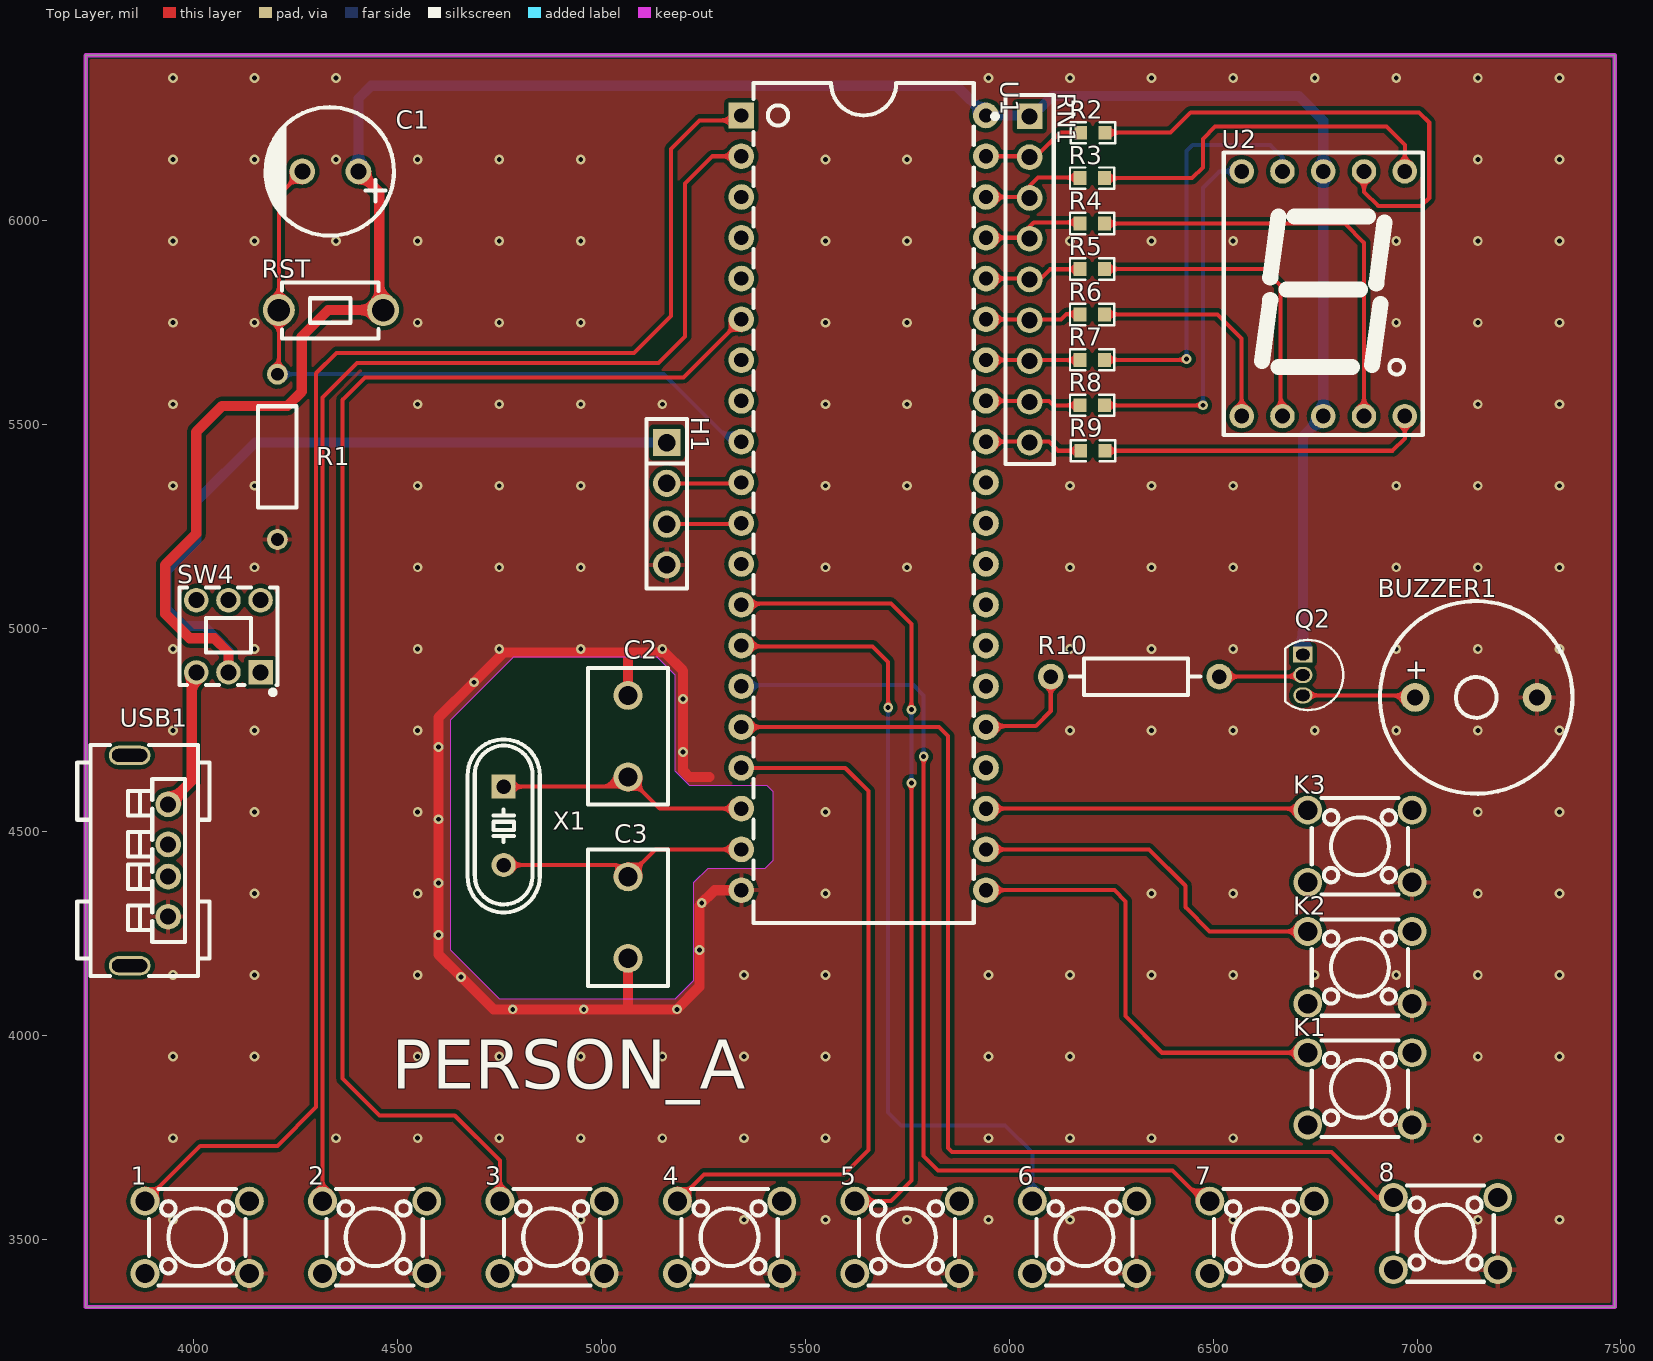
[diagram p0: Top Layer view]
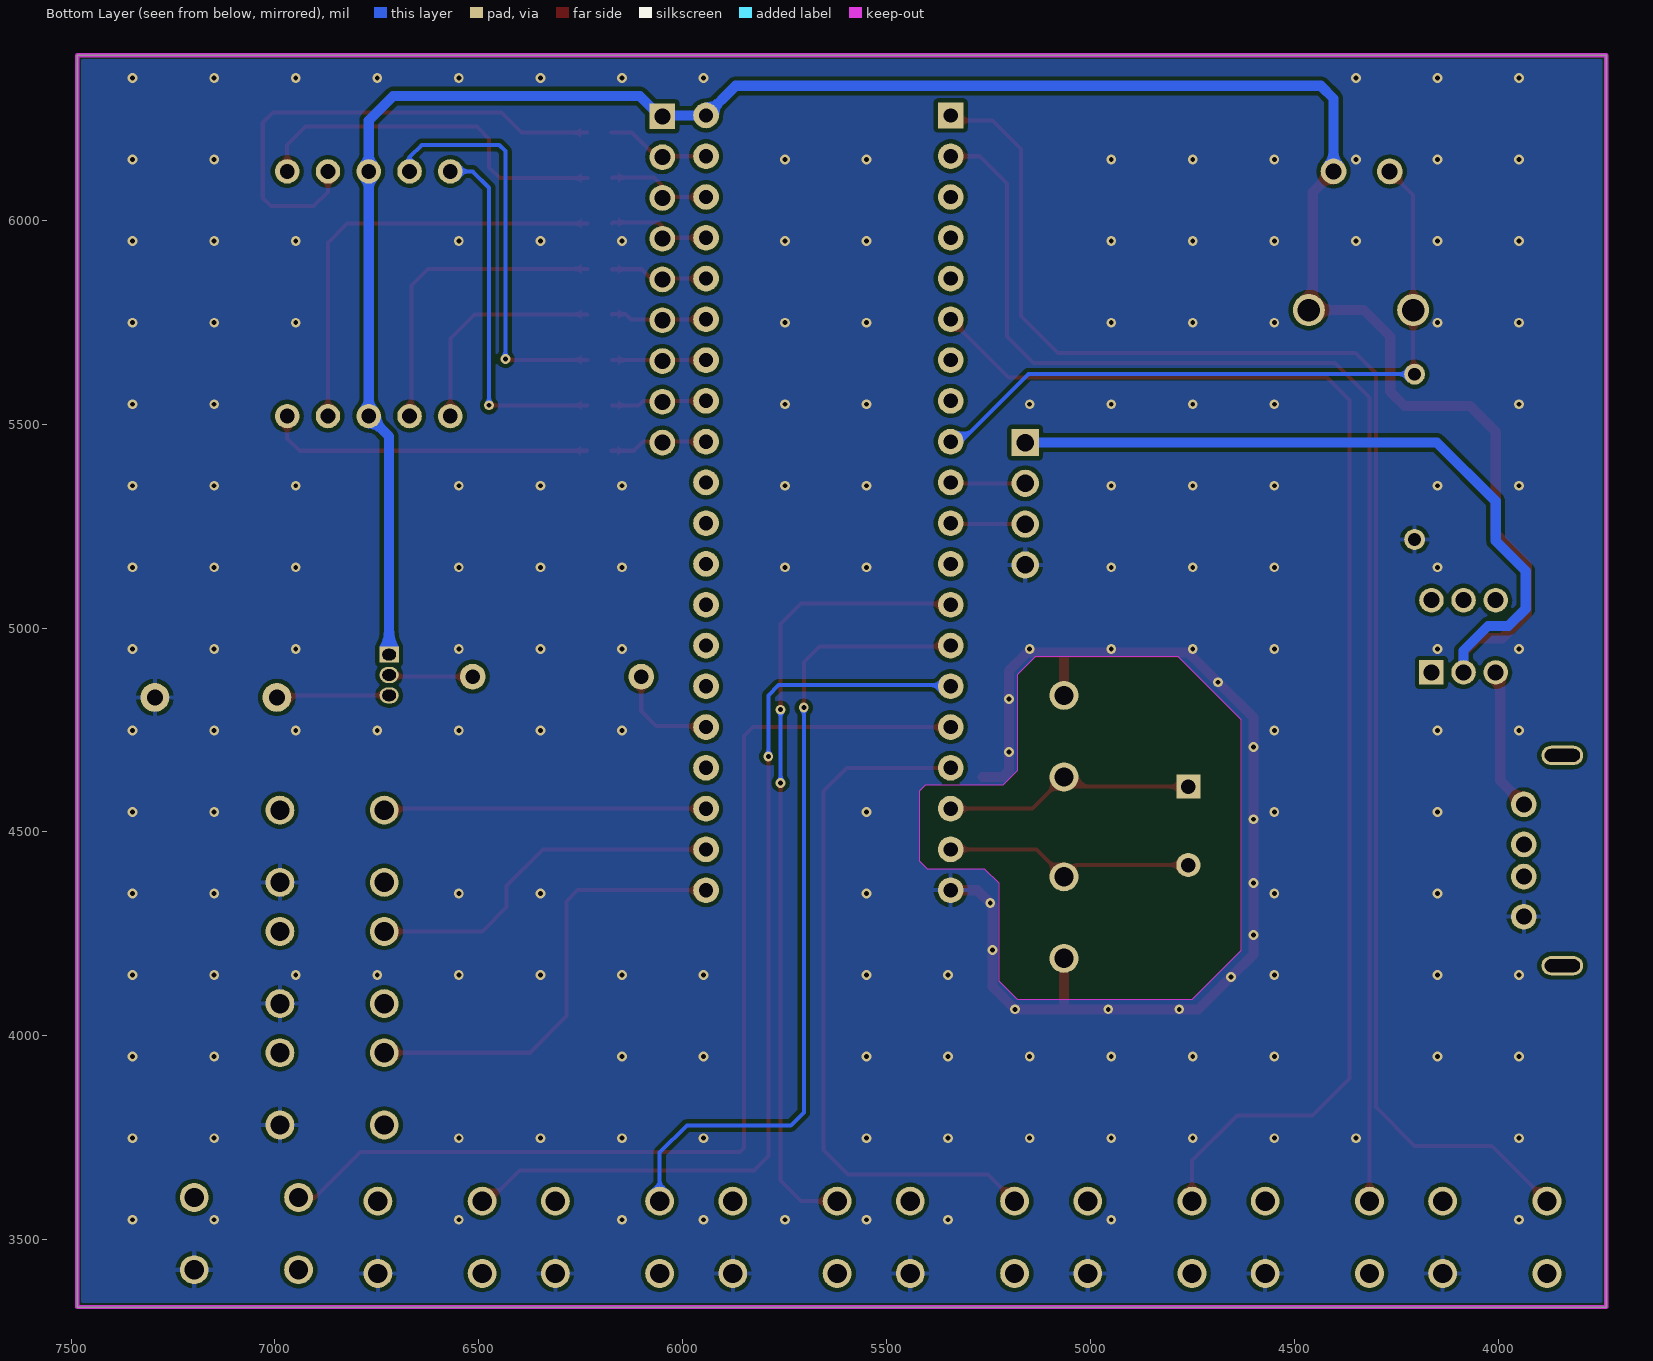
[diagram p1: Bottom Layer view, seen from below]
# Altium PCB MISC49928.pcbdoc
Units mil, origin at the board's own origin, x right, y up, seen from the top; angles counter-clockwise.
Board outline 3750 x 3070 mil, 2 copper layers (Top Layer, Bottom Layer), stack 62.206 mil thick; 34 components, 38 nets, 154 pads, 181 vias.

## Layer stack, top to bottom
Top Solder Mask Layer: solder mask 0.394, Dk 3.3
Top Layer: signal copper 1.379
Dielectric1: surface 59.449, FR4, Dk 4.5
Bottom Layer: signal copper 1.378
Bottom Solder Mask Layer: solder mask 0.394, Dk 3.3

## Board outline
3735,6405 3735,3335 7485,3335 7485,6405

## Design rules (kind name [scope] priority, off if disabled: settings)
BoardOutlineClearance copperThickness2oz_1 [All] p2 off: genericclearance=7.99 ignorepadtopadclearanceinfootprint=FALSE except(0: Arc-SplitContinuation Track-SplitContinuation SMDPad-SplitContinuation THPad-SplitContinuation Via-SplitContinuation Fill-SplitContinuation Region-SplitContinuation Poly-SplitContinuation Text-SplitContinuation Hole-SplitContinuation; 5.98: Arc-CutoutEdge SMDPad-CutoutEdge THPad-CutoutEdge Via-CutoutEdge Fill-CutoutEdge Region-CutoutEdge Text-CutoutEdge; 6.93: Hole-OutlineEdge Hole-CutoutEdge; 10: Poly-OutlineEdge Poly-CutoutEdge; 11.81: Arc-OutlineEdge Track-OutlineEdge SMDPad-OutlineEdge THPad-OutlineEdge Via-OutlineEdge Fill-OutlineEdge Region-OutlineEdge Text-OutlineEdge Track-CutoutEdge)
BoardOutlineClearance copperThickness1oz_1 [All] p4: genericclearance=4.02 ignorepadtopadclearanceinfootprint=FALSE except(0: Arc-SplitContinuation Track-SplitContinuation SMDPad-SplitContinuation THPad-SplitContinuation Via-SplitContinuation Fill-SplitContinuation Region-SplitContinuation Poly-SplitContinuation Text-SplitContinuation Hole-SplitContinuation; 6: SMDPad-CutoutEdge THPad-CutoutEdge Via-CutoutEdge Fill-CutoutEdge Region-CutoutEdge Text-CutoutEdge; 6.93: Hole-OutlineEdge Hole-CutoutEdge; 10: Poly-OutlineEdge Poly-CutoutEdge; 11.8: Arc-OutlineEdge Track-OutlineEdge SMDPad-OutlineEdge THPad-OutlineEdge Via-OutlineEdge Fill-OutlineEdge Region-OutlineEdge Text-OutlineEdge; 11.81: Arc-CutoutEdge Track-CutoutEdge)
Clearance copperThickness2oz [All] p1 off: gap=7.99 ignorepadtopadclearanceinfootprint=FALSE except(5.98: SMDPad-Track SMDPad-SMDPad THPad-Track SMDPad-THPad THPad-THPad Track-Via SMDPad-Via THPad-Via Via-Via Fill-Track Region-Track Fill-SMDPad Region-SMDPad Fill-THPad Region-THPad Fill-Via Region-Via Fill-Fill Fill-Region Region-Region Arc-Track Arc-SMDPad Arc-THPad Arc-Via Fill-Arc Region-Arc Arc-Arc Text-Track SMDPad-Text Text-THPad Text-Via Fill-Text Region-Text Arc-Text Text-Text; 6.93: Hole-Track Hole-SMDPad Hole-THPad Hole-Via Fill-Hole Region-Hole Hole-Arc Hole-Text; 10: Poly-Track Poly-SMDPad Poly-THPad Poly-Via Poly-Fill Poly-Region Poly-Poly Poly-Arc Poly-Text Poly-Hole)
Clearance copperThickness1oz [All] p3: gap=4.02 ignorepadtopadclearanceinfootprint=FALSE except(5.98: SMDPad-Track SMDPad-SMDPad THPad-Track SMDPad-THPad THPad-THPad Track-Via SMDPad-Via THPad-Via Via-Via Fill-Track Region-Track Fill-SMDPad Region-SMDPad Fill-THPad Region-THPad Fill-Via Region-Via Fill-Fill Fill-Region Region-Region; 6: Arc-Track Arc-SMDPad Arc-THPad Arc-Via Fill-Arc Region-Arc Arc-Arc Text-Track SMDPad-Text Text-THPad Text-Via Fill-Text Region-Text Arc-Text Text-Text; 6.93: Hole-Track Hole-SMDPad Hole-THPad Hole-Via Fill-Hole Region-Hole Hole-Arc Hole-Text; 10: Poly-Track Poly-SMDPad Poly-THPad Poly-Via Poly-Fill Poly-Region Poly-Poly Poly-Arc Poly-Text Poly-Hole)
DiffPairsRouting differentialPair [All] p1: maxlimit=6 minlimit=6 mostfreqgap=6 toplayer_minwidth=5 toplayer_prefwidth=10 toplayer_maxwidth=100 toplayer_mingap=6 toplayer_prefgap=6 toplayer_maxgap=6 bottomlayer_minwidth=5 bottomlayer_prefwidth=10 bottomlayer_maxwidth=100 bottomlayer_mingap=6 bottomlayer_prefgap=6 bottomlayer_maxgap=6 maxuncoupledlength=10
HoleToHoleClearance otherClearance [All] p1: gap=11.81 allowstackedmicrovias=TRUE
Length netLength [All] p1: minlimit=0 maxlimit=0
MatchedLengths netLengthTolerance [All] p1: tolerance=1000
PasteMaskExpansion pasteMaskExpansion [All] p1: expansion=0
PlaneConnect innerPlane [All] p1: planeconnectstyle=Relief reliefexpansion=20 reliefentries=4 reliefconductorwidth=10 reliefairgap=10
PolygonConnect copperRegion [(InNet('GND'))] p1: connectstyle=Relief reliefconductorwidth=10 reliefentries=4 polygonreliefangle="90 Angle" airgapwidth=10 via.connectstyle=Relief via.reliefconductorwidth=10 via.reliefentries=4 via.polygonreliefangle="90 Angle" via.airgapwidth=10
RoutingVias viaSize [All] p1: holewidth=12.01 width=24.02 viastyle="Through Hole" minholewidth=11.81 minwidth=19.68 maxholewidth=248.03 maxwidth=393.7
SolderMaskExpansion solderMaskExpansion [IsVia] p1: expansion=-1000 istentingtop=TRUE
SolderMaskExpansion solderMaskExpansion [All] p2: expansion=2 istentingtop=FALSE
Width copperThickness2oz_2 [All] p1 off: maxlimit=100 minlimit=8 preferedwidth=10
Width copperThickness1oz_2 [All] p2: maxlimit=100 minlimit=5 preferedwidth=10

## Components (designator, comment, footprint, x,y, rotation, side; value= is the part's Value field where it differs from the comment)
1 "TS665CJ" SW-TH_4P-L6.0-W6.0-P4.50-LS6.5 4008.28,3505.92 r0 top
2 "TS665CJ" SW-TH_4P-L6.0-W6.0-P4.50-LS6.5 4443.53,3505.92 r0 top
3 "TS665CJ" SW-TH_4P-L6.0-W6.0-P4.50-LS6.5 4878.77,3505.92 r0 top
4 "TS665CJ" SW-TH_4P-L6.0-W6.0-P4.50-LS6.5 5314.02,3505.92 r0 top
5 "TS665CJ" SW-TH_4P-L6.0-W6.0-P4.50-LS6.5 5749.26,3505.92 r0 top
6 "TS665CJ" SW-TH_4P-L6.0-W6.0-P4.50-LS6.5 6184.51,3505.92 r0 top
7 "TS665CJ" SW-TH_4P-L6.0-W6.0-P4.50-LS6.5 6619.75,3505.92 r0 top
8 "TS665CJ" SW-TH_4P-L6.0-W6.0-P4.50-LS6.5 7070,3515 r0 top
BUZZER1 "2.4kHz" BUZ-TH_BD12.0-P7.60-D0.6-FD 7145,4830 r0 top
C1 "10uF" CAP-TH_BD8.0-P3.50-D0.6-FD 4335,6120 r180 top
C2 "30pF" CAP-TH_L8.5-W5.0-P5.00-D1.2 5065,4735 r270 top
C3 "30pF" CAP-TH_L8.5-W5.0-P5.00-D1.2 5065,4290 r90 top
H1 "" HDR-TH_4P-P2.54-V-F 5160,5305 r270 top
K1 "TS665CJ" SW-TH_4P-L6.0-W6.0-P4.50-LS6.5 6860,3870 r0 top
K2 "TS665CJ" SW-TH_4P-L6.0-W6.0-P4.50-LS6.5 6860,4167.5 r0 top
K3 "TS665CJ" SW-TH_4P-L6.0-W6.0-P4.50-LS6.5 6860,4465 r0 top
Q2 "S8550" TO-92-3_L4.5-W3.5-P1.27-L 6720,4885 r270 top
R1 "10kΩ" RES-TH_BD2.4-L6.3-P10.30-D0.6 4205,5420 r90 top
R2 "470" R0603 6205,6215 r0 top
R3 "470" R0603 6203.43,6103.57 r0 top
R4 "470" R0603 6203.43,5992.14 r0 top
R5 "470" R0603 6203.43,5880.71 r0 top
R6 "470" R0603 6203.43,5769.29 r0 top
R7 "470" R0603 6203.43,5657.86 r0 top
R8 "470" R0603 6203.43,5546.43 r0 top
R9 "470" R0603 6205,5435 r0 top
R10 "4.7K" RES-TH_BD2.2-L6.5-P10.50-D0.6 6308.43,4880.92 r0 top
RN1 "-" RES-ARRAY-TH_9P-P2.54-D1.0 6050,5855 r270 top
RST "" Key_TH_3.5x6x4.3 4330,5780 r0 top
SW4 "5.8 ZSGT" SW-TH_5.8ZSGT 4085,4980 r0 top
U1 "STC89C52RC-40I-PDIP40" DIP-40_L52.0-W13.7-P2.54-LS15.2-BL 5642.86,5307.29 r270 top
U2 "TDSR1360" LED-SEG-TH_10P-L17.6-W12.4-P2.54-S15.24-BL 6770,5820 r0 top
USB1 "AF 180°ZJB13.7" USB-A-TH_AF-ZJB13.7 3890,4430 r270 top
X1 "12MHz" HC-49US_L11.5-W4.5-P4.88 4760,4515 r270 top

## Footprints (in the part's own frame and the unit in brackets; to place one, negate y for a bottom-side part, rotate by r counter-clockwise, add the part's x,y. Pads: shape width x height; smd on the part's side, far side on the other; paste and mask are expansions set on the pad)
BUZ-TH_BD12.0-P7.60-D0.6-FD [mm]
  round 1.8 hole 1: 1(-3.8,0) 2(3.8,0)
  silkscreen extent -6,-6 6,6
CAP-TH_BD8.0-P3.50-D0.6-FD [mm]
  round 1.6 hole 1: 1(-1.75,0) 2(1.75,0)
  silkscreen extent -3.96,-4 4.04,4
CAP-TH_L8.5-W5.0-P5.00-D1.2 [mm]
  round 1.8 hole 1.2: 1(-2.54,0) 2(2.54,0)
  silkscreen extent -4.25,-2.5 4.25,2.5
DIP-40_L52.0-W13.7-P2.54-LS15.2-BL [mil]
  rect 63x63 hole 35: 1(-950,-300)
  round 63 hole 35: 2(-850,-300) 3(-750,-300) 4(-650,-300) 5(-550,-300) 6(-450,-300) 7(-350,-300) 8(-250,-300) 9(-150,-300) 10(-50,-300) 11(50,-300) 12(150,-300) 13(250,-300) 14(350,-300) 15(450,-300) 16(550,-300) 17(650,-300) 18(750,-300) 19(850,-300) 20(950,-300) 21(950,300) 22(850,300) 23(750,300) 24(650,300) 25(550,300) 26(450,300) 27(350,300) 28(250,300) 29(150,300) 30(50,300) 31(-50,300) 32(-150,300) 33(-250,300) 34(-350,300) 35(-450,300) 36(-550,300) 37(-650,300) 38(-750,300) 39(-850,300) 40(-950,300)
  silkscreen extent -1030,-270 1030,270
HC-49US_L11.5-W4.5-P4.88 [mm]
  rect 1.5x1.5 hole 0.9: 1(-2.44,0)
  round 1.5 hole 0.9: 2(2.44,0)
  silkscreen extent -5.39,-2.25 5.39,2.25
HDR-TH_4P-P2.54-V-F [mm]
  rect 1.7x1.7 hole 1.1: 1(-3.81,0)
  round 1.7 hole 1.1: 2(-1.27,0) 3(1.27,0) 4(3.81,0)
  silkscreen extent -5.29,-1.27 5.29,1.27
Key_TH_3.5x6x4.3 [mil]
  round 78.7 hole 55.1 paste+0 mask+2: A(-121.44,0) B(134.46,0)
  silkscreen extent -114,-70 123,68
LED-SEG-TH_10P-L17.6-W12.4-P2.54-S15.24-BL [mil]
  round 60 hole 36: 1(-200,-300) 2(-100,-300) 3(0,-300) 4(100,-300) 5(200,-300) 6(200,300) 7(100,300) 8(0,300) 9(-100,300) 10(-200,300)
  silkscreen extent -244,-346 244,346
R0603 [mil]
  rect 31.75x34.02 smd paste-3937.01 mask+2: 1(-29.66,0) 2(29.66,0)
  silkscreen extent -55,-26 55,26
RES-ARRAY-TH_9P-P2.54-D1.0 [mm]
  rect 1.6x1.6 hole 1: 1(-10.16,0)
  round 1.6 hole 1: 2(-7.62,0) 3(-5.08,0) 4(-2.54,0) 5(0,0) 6(2.54,0) 7(5.08,0) 8(7.62,0) 9(10.16,0)
  silkscreen extent -11.5,-2.31 11.5,1.5
RES-TH_BD2.2-L6.5-P10.50-D0.6 [mm]
  round 1.6 hole 0.914: 1(-5.25,0) 2(5.25,0)
  silkscreen extent -4.06,-1.14 4.06,1.14
RES-TH_BD2.4-L6.3-P10.30-D0.6 [mm]
  round 1.3 hole 0.8: 1(-5.15,0) 2(5.15,0)
  silkscreen extent -3.15,-1.2 3.15,1.2
SW-TH_4P-L6.0-W6.0-P4.50-LS6.5 [mm]
  round 1.8 hole 1.2: 1(-3.25,2.25) 2(3.25,2.25) 3(-3.25,-2.25) 4(3.25,-2.25)
  silkscreen extent -3,-3 3,3
SW-TH_5.8ZSGT [mm]
  rect 1.524x1.524 hole 1: 1(2,-2.25)
  round 1.524 hole 1: 2(0,-2.25) 3(-2,-2.25) 4(2,2.25) 5(0,2.25) 6(-2,2.25)
  silkscreen extent -3.05,-3.64 3.05,3.05
TO-92-3_L4.5-W3.5-P1.27-L [mm]
  rect 1x1.2 hole 0.7 slot 0.85 at 90 deg: 1(-1.27,0)
  oval 1x1.2 hole 0.7 slot 0.85 at 90 deg: 2(0,0) 3(1.27,0)
  silkscreen extent -2.19,-1.1 2.19,2.52
USB-A-TH_AF-ZJB13.7 [mm]
  round 1.6 hole 1: 1(-3.5,1.2) 2(-1,1.2) 3(1,1.2) 4(3.5,1.2)
  oval 1.2x2.6 hole 0.8 slot 2.2 at 90 deg: 5(-6.55,-1.2) 5(6.55,-1.2)
  silkscreen extent -7.2,-4.47 7.2,3.76

## Via types
v1: diameter 24.02, hole 12, Top Layer to Bottom Layer, 181 vias

## Nets (pads, with @x,y where several pads share a name; then routed paths per layer and width w, separated by ;. In a path a pad name is that pad's centre, name@x,y a point inside that pad or via, vN(x,y) a via of type N, cw(c..) or ccw(c..) an arc to the next point about the centre after c; other vN are vias at no path point)
$1N19: R2.1 RN1.2 U1.39 | length 256.4
  Top Layer w10: U1.39 6067.29,6157.29 6125,6215 R2.1
$1N20: R3.1 RN1.3 U1.38 | length 251.3
  Top Layer w10: U1.38 6022.29,6057.29 6070,6105 6172.34,6105 R3.1
$1N21: R4.1 RN1.4 U1.37 | length 247.7
  Top Layer w10: U1.37 6022.29,5957.29 6060,5995 6170.91,5995 R4.1
$1N22: R5.1 RN1.5 U1.36 | length 240.6
  Top Layer w10: U1.36 6077.29,5857.29 6100,5880 6173.06,5880 R5.1
$1N23: R6.1 RN1.6 U1.35 | length 236.5
  Top Layer w10: U1.35 6127.29,5757.29 6140,5770 6173.06,5770 R6.1
$1N24: R9.1 RN1.9 U1.32 | length 241.7
  Top Layer w10: U1.32 6097.71,5457.29 6120,5435 R9.1
$1N25: R8.1 RN1.8 U1.33 | length 235.4
  Top Layer w10: U1.33 6097.71,5557.29 6108.57,5546.43 R8.1
$1N26: R7.1 RN1.7 U1.34 | length 231.1
  Top Layer w10: U1.34 6173.2,5657.29 R7.1
$1N27: R10.1 U1.25 | length 259.4
  Top Layer w10: U1.25 5945.57,4760 6065,4760 6101.73,4796.73 R10.1
$1N28: Q2.2 R10.2 | length 206.6
  Top Layer w10: R10.2 6715.92,4880.92 Q2.2
$1N29: BUZZER1.1 Q2.3 | length 277.5
  Top Layer w10: Q2.3 6990.4,4835 BUZZER1.1
$1N67: SW4.3 USB1.1 | length 352.2
  Top Layer w25: USB1.1 3995,4625.55 3995,4880.16 SW4.3
$1N90: H1.2 U1.10 | length 183.8
  Top Layer w10: H1.2 5340.57,5355 U1.10
$1N91: H1.3 U1.11 | length 183.8
  Top Layer w10: H1.3 5340.57,5255 U1.11
A: R2.2 U2.7 | length 1244.2
  Top Layer w10: R2.2 6395,6215 6445,6265 7005,6265 7030,6240 7030,6055 7010,6035 6905,6035 6870,6070 U2.7
B: R3.2 U2.6 | length 913.9
  Top Layer w10: R3.2 6448.57,6103.57 6475,6130 6475,6200 6505,6230 6925,6230 6970,6185 U2.6
C: R4.2 U2.4 | length 1081.4
  Top Layer w10: R4.2 6822.86,5992.14 6870,5945 U2.4
D: R5.2 U2.2 | length 770.8
  Top Layer w10: R5.2 6624.29,5880.71 6665,5840 6665,5525 U2.2
E: R6.2 U2.1 | length 551.5
  Top Layer w10: R6.2 6510.71,5769.29 6570,5710 U2.1
F: R7.2 U2.9 | length 1001.4
  Top Layer w10: R7.2 6432.86,5657.86 v1(6435,5660)
  Bottom Layer w10: v1(6435,5660) 6435,6170 6450,6185 6640,6185 6670,6155 U2.9
G: R8.2 U2.10 | length 887.1
  Top Layer w10: R8.2 v1(6475,5546.43)
  Bottom Layer w10: v1(6475,5546.43) 6475,6080 6515,6120 U2.10
GND: 1.4 2.4 3.4 4.4 5.4 6.4 7.4 8.4 BUZZER1.2 C2.1 C3.1 H1.4 K1.4 K2.4 K3.4 R1.1 U1.20 USB1.4 | length 2850.2
  Top Layer w25: 5065,4065.04 C3.1 ; C2.1 5065,4934.92 5070.08,4940 ; 5265,4635 5215,4635 5200,4650 v1(5200,4696.11) v1(5200,4826.14) 5200,4895 5155,4940 5070.08,4940 ; U1.20 5277.29,4357.29 5240,4320 v1(5240,4210.77) 5240,4120 v1(5185,4065) 5064.96,4065 v1(4956.42,4065) v1(4782.36,4065) 4735,4065 v1(4655.59,4144.41) 4600,4200 v1(4600,4247.63) v1(4600,4375) v1(4600,4531.26) v1(4600,4708.39) 4600,4780 v1(4687.12,4867.12) 4760,4940 5070.08,4940
  other v1: 3949.1,3549.1 4949.1,3549.1 5349.1,3549.1 5549.1,3549.1 5749.1,3549.1 5949.1,3549.1 6149.1,3549.1 6549.1,3549.1 7149.1,3549.1 7349.1,3549.1 3949.1,3749.1 4349.1,3749.1 4549.1,3749.1 4749.1,3749.1 4949.1,3749.1 5149.1,3749.1 5349.1,3749.1 5549.1,3749.1 5949.1,3749.1 6149.1,3749.1 6349.1,3749.1 6549.1,3749.1 7149.1,3749.1 7349.1,3749.1 3949.1,3949.1 4149.1,3949.1 4549.1,3949.1 4749.1,3949.1 4949.1,3949.1 5149.1,3949.1 5349.1,3949.1 5549.1,3949.1 5949.1,3949.1 6149.1,3949.1 7149.1,3949.1 7349.1,3949.1 3949.1,4149.1 4149.1,4149.1 4549.1,4149.1 5349.1,4149.1 5549.1,4149.1 5949.1,4149.1 6149.1,4149.1 6349.1,4149.1 6549.1,4149.1 6749.1,4149.1 6949.1,4149.1 7149.1,4149.1 7349.1,4149.1 5245.82,4325.82 4149.1,4349.1 4549.1,4349.1 5549.1,4349.1 6349.1,4349.1 6549.1,4349.1 7149.1,4349.1 7349.1,4349.1 4149.1,4549.1 4549.1,4549.1 5549.1,4549.1 7149.1,4549.1 7349.1,4549.1 3949.1,4749.1 4149.1,4749.1 4549.1,4749.1 6149.1,4749.1 6349.1,4749.1 6549.1,4749.1 6749.1,4749.1 6949.1,4749.1 7149.1,4749.1 7349.1,4749.1 3949.1,4949.1 4149.1,4949.1 4549.1,4949.1 4749.1,4949.1 4949.1,4949.1 5149.1,4949.1 6149.1,4949.1 6349.1,4949.1 6549.1,4949.1 6949.1,4949.1 7149.1,4949.1 7349.1,4949.1 4149.1,5149.1 4549.1,5149.1 4749.1,5149.1 4949.1,5149.1 5549.1,5149.1 5749.1,5149.1 6149.1,5149.1 6349.1,5149.1 6549.1,5149.1 6949.1,5149.1 7149.1,5149.1 7349.1,5149.1 3949.1,5349.1 4149.1,5349.1 4549.1,5349.1 4749.1,5349.1 4949.1,5349.1 5549.1,5349.1 5749.1,5349.1 6149.1,5349.1 6349.1,5349.1 6549.1,5349.1 6949.1,5349.1 7149.1,5349.1 7349.1,5349.1 3949.1,5549.1 4549.1,5549.1 4749.1,5549.1 4949.1,5549.1 5149.1,5549.1 5549.1,5549.1 5749.1,5549.1 7149.1,5549.1 7349.1,5549.1 3949.1,5749.1 4149.1,5749.1 4549.1,5749.1 4749.1,5749.1 4949.1,5749.1 5549.1,5749.1 5749.1,5749.1 6949.1,5749.1 7149.1,5749.1 7349.1,5749.1 3949.1,5949.1 4149.1,5949.1 4349.1,5949.1 4549.1,5949.1 4749.1,5949.1 4949.1,5949.1 5549.1,5949.1 5749.1,5949.1 6149.1,5949.1 6349.1,5949.1 6549.1,5949.1 6949.1,5949.1 7149.1,5949.1 7349.1,5949.1 3949.1,6149.1 4149.1,6149.1 4349.1,6149.1 4549.1,6149.1 4749.1,6149.1 4949.1,6149.1 5549.1,6149.1 5749.1,6149.1 7149.1,6149.1 7349.1,6149.1 3949.1,6349.1 4149.1,6349.1 4349.1,6349.1 5949.1,6349.1 6149.1,6349.1 6349.1,6349.1 6549.1,6349.1 6749.1,6349.1 6949.1,6349.1 7149.1,6349.1 7349.1,6349.1
H: R9.2 U2.5 | length 802.8
  Top Layer w10: R9.2 6940,5435 6970,5465 U2.5
P1.0: 1.1 U1.1 | length 3860.1
  Top Layer w10: 1.1 4015.84,3730 4205,3730 4300,3825 4300,5625 4350,5675 5080,5675 5170,5765 5170,6175 5240,6245 5330.57,6245 U1.1
P1.1: 2.1 U1.2 | length 3463.1
  Top Layer w10: 2.1 4315.58,5565.58 4400,5650 5140,5650 5205,5715 5205,6090 5272.29,6157.29 U1.2
P1.4: 3.1 U1.6 | length 3293.3
  Top Layer w10: 3.1 4750.82,3694.18 4640,3805 4455,3805 4365,3895 4365,5560 4420,5615 5200.57,5615 U1.6
P2.0: K1.1 U1.21 | length 1119.3
  Top Layer w10: U1.21 6257.71,4357.29 6285,4330 6285,4048.48 6374.9,3958.58 K1.1
P2.1: K2.1 U1.22 | length 903.4
  Top Layer w10: U1.22 6342.71,4457.29 6431.9,4368.1 6431.9,4315.49 6491.31,4256.08 K2.1
P2.2: K3.1 U1.23 | length 790.7
  Top Layer w10: U1.23 6728.34,4557.29 K3.1
P3.3: 5.1 U1.13 | length 1963.6
  Top Layer w10: U1.13 5345.57,5060 5710,5060 5760,5010 v1(5760,4800) ; 5.1 5709.5,3594.5 5760,3645 v1(5760,4620)
  Bottom Layer w10: v1(5760,4620) v1(5760,4800)
P3.4: 6.1 U1.14 | length 1995.2
  Top Layer w10: U1.14 5345.15,4955 5665,4955 5703.02,4916.98 v1(5703.02,4805)
  Bottom Layer w10: v1(5703.02,4805) 5703.02,3811.97 5735,3780 5990,3780 6056.56,3713.44 6.1
P3.5: 7.1 U1.15 | length 2336.2
  Top Layer w10: v1(5790,4685) 5790,3705 5825,3670 6400,3670 6475.5,3594.5 7.1
  Bottom Layer w10: U1.15 5345.57,4860 5765,4860 5790,4835 v1(5790,4685)
P3.6: 8.1 U1.16 | length 2668.7
  Top Layer w10: U1.16 5827.71,4757.29 5850,4735 5850,3725 5860,3715 6790,3715 6901.42,3603.58 8.1
P3.7: 4.1 U1.17 | length 1736.8
  Top Layer w10: 4.1 5251.57,3660 5595,3660 5655,3720 5655,4600 5597.71,4657.29 U1.17
RST: C1.2 R1.2 RST.A U1.9 | length 1728.9
  Top Layer w10: R1.2 4208.56,5626.32 RST.A 4208.56,6062.46 C1.2
  Bottom Layer w10: R1.2 5152.24,5622.76 5317.71,5457.29 U1.9
VCC: C1.1 H1.1 Q2.1 RN1.1 RST.B SW4.2 U1.40 U2.3 U2.8 | length 7462.4
  Top Layer w25: SW4.2 4085,4940 4050,4975 3990,4975 3930,5035 3930,5155 4006.26,5231.26 4006.26,5481.26 4070,5545 4230,5545 4265,5580 4265,5715 4330,5780 RST.B@4455,5780 ; C1.1 4455,6068.9 RST.B@4455,5780 ; RST.B RST.B@4455,5780
  Bottom Layer w25: SW4.2 4085,4945 4025,5005 3975,5005 3932.5,5047.5 3932.5,5140 4006.26,5213.76 4006.26,5311.26 4150,5455 H1.1 ; C1.1 4403.9,6298.9 4435,6330 5870.15,6330 U1.40 6057.29,6257.29 6105,6305 6710,6305 6770,6245 U2.8 U2.3 6720,5470 Q2.1
X1: C3.2 U1.19 X1.2 | length 622.7
  Top Layer w10: X1.2 5036.06,4418.94 C3.2 5132.29,4457.29 U1.19
X2: C2.2 U1.18 X1.1 | length 625
  Top Layer w10: X1.1 5041.06,4611.06 C2.2 5142.71,4557.29 U1.18
pads on no net: 1.2 1.3 2.2 2.3 3.2 3.3 4.2 4.3 5.2 5.3 6.2 6.3 7.2 7.3 8.2 8.3 K1.2 K1.3 K2.2 K2.3 K3.2 K3.3 SW4.1 SW4.4 SW4.5 SW4.6 U1.3 U1.4 U1.5 U1.7 U1.8 U1.12 U1.24 U1.26 U1.27 U1.28 U1.29 U1.30 U1.31 USB1.2 USB1.3 USB1.5

## Polygon pours and split planes (outlines as drawn)
GND on Bottom Layer (solid, remove dead copper, pour order 2): 3380,6890 3380,3000 8450,3000 8450,6890
GND on Top Layer (solid, remove dead copper, pour order 0): 3000,6920 3000,3150 8150,3150 8150,6920

## Keep-outs
Board Outline Layer:
  region: 5135,4930 5180,4885 5180,4650 5215,4615 5405,4615 5420,4600 5420,4430 5400,4410 5260,4410 5225,4375 5225,4135 5180,4090 4750,4090 4630,4210 4630,4775 4785,4930
  lines w10: 3735,3335 3735,6405 7485,6405 7485,3335 3735,3335

## Other copper
Top Layer:
  drawing of 76 lines, arcs and shapes, not listed
Bottom Layer:
  region net VCC: 4391.4,6162.88 4416.4,6162.88 4416.49,6161.22 4416.74,6159.55 4417.68,6156.24 4419.06,6153.01 4420.74,6149.94 4422.57,6147.11 4424.41,6144.6 4427.52,6140.83 4380.28,6140.83 4383.39,6144.6 4385.23,6147.11 4387.06,6149.94 4388.74,6153.01 4390.12,6156.24 4391.06,6159.55 4391.31,6161.22
  region net VCC: 6707.5,4992.19 6732.5,4992.19 6732.82,4985.58 6733.77,4979.05 6735.34,4972.63 6737.52,4966.39 6740.29,4960.39 6743.62,4954.69 6696.38,4954.69 6699.71,4960.39 6702.48,4966.39 6704.66,4972.63 6706.23,4979.05 6707.18,4985.58 6707.5,4992.19
  region net RST: 4239.84,5627.76 4239.84,5617.76 4238.5,5617.63 4237.15,5617.27 4235.82,5616.71 4234.5,5615.97 4231.93,5614.07 4229.48,5611.8 4225.16,5607.06 4223.39,5605.05 4221.93,5603.57 4221.93,5641.95 4223.39,5640.48 4225.16,5638.46 4229.48,5633.72 4231.93,5631.45 4234.5,5629.55 4235.82,5628.81 4237.15,5628.25 4238.5,5627.89
  region net VCC: 5903.7,6278.78 5921.37,6296.45 5922.61,6295.34 5923.97,6294.34 5926.98,6292.66 5930.24,6291.35 5933.59,6290.37 5936.89,6289.66 5939.96,6289.19 5944.83,6288.73 5911.42,6255.32 5910.96,6260.19 5910.49,6263.26 5909.78,6266.56 5908.8,6269.91 5907.49,6273.17 5905.81,6276.18 5904.81,6277.54
  region net RST: 5308.43,5459.5 5296.64,5485.43 5297.95,5484.36 5299.51,5483.47 5301.29,5482.75 5303.24,5482.2 5305.34,5481.8 5307.54,5481.54 5312.09,5481.4 5316.58,5481.7 5320.73,5482.34 5324.22,5483.26 5326.74,5484.35 5318.02,5437.91 5317.03,5439.65 5316.18,5441.98 5314.47,5447.77 5313.44,5450.91 5312.15,5454.02 5310.51,5456.94 5309.53,5458.27
  region net P3.5: 5383.64,4865 5387.7,4855 5386.04,4854.83 5384.39,4854.34 5382.74,4853.57 5381.1,4852.56 5379.49,4851.34 5377.92,4849.97 5374.89,4846.87 5372.08,4843.57 5369.57,4840.38 5367.4,4837.6 5365.65,4835.55 5361.59,4882.62 5363.47,4880.9 5365.71,4878.45 5371.01,4872.55 5373.98,4869.69 5377.11,4867.28 5378.71,4866.34 5380.34,4865.62 5381.98,4865.16
  region net G: 6529.16,6115 6529.16,6125 6530.73,6125.16 6532.3,6125.6 6533.86,6126.31 6535.41,6127.23 6538.41,6129.58 6541.27,6132.39 6543.93,6135.37 6546.33,6138.24 6548.42,6140.71 6550.16,6142.5 6550.16,6097.5 6548.42,6099.29 6546.33,6101.76 6543.93,6104.63 6541.27,6107.61 6538.41,6110.42 6535.41,6112.77 6533.86,6113.69 6532.3,6114.4 6530.73,6114.84
  region net F: 6665,6155 6675,6155 6675.16,6153.87 6675.63,6152.75 6676.35,6151.65 6677.3,6150.56 6679.73,6148.46 6682.6,6146.45 6688.47,6142.82 6690.87,6141.24 6692.5,6139.84 6647.5,6139.84 6649.13,6141.24 6651.53,6142.82 6657.4,6146.45 6660.27,6148.46 6662.7,6150.56 6663.65,6151.65 6664.37,6152.75 6664.84,6153.87
  region net VCC: 6782.5,6079.16 6757.5,6079.16 6757.42,6080.74 6757.2,6082.33 6756.37,6085.49 6755.15,6088.57 6753.65,6091.5 6752.02,6094.19 6750.36,6096.59 6747.5,6100.16 6792.5,6100.16 6789.64,6096.59 6787.98,6094.19 6786.35,6091.5 6784.85,6088.57 6783.63,6085.49 6782.8,6082.33 6782.58,6080.74
  region net VCC: 6757.5,6160.84 6782.5,6160.84 6782.58,6159.26 6782.8,6157.67 6783.63,6154.51 6784.85,6151.43 6786.35,6148.5 6787.98,6145.81 6789.64,6143.41 6792.5,6139.84 6747.5,6139.84 6750.36,6143.41 6752.02,6145.81 6753.65,6148.5 6755.15,6151.43 6756.37,6154.51 6757.2,6157.67 6757.42,6159.26
  region net VCC: 6749.96,5482.28 6732.28,5499.96 6733.34,5501.13 6734.31,5502.42 6735.96,5505.24 6737.28,5508.28 6738.29,5511.4 6739.04,5514.47 6739.56,5517.33 6740.06,5521.88 6771.88,5490.06 6767.33,5489.56 6764.47,5489.04 6761.4,5488.29 6758.28,5487.28 6755.24,5485.96 6752.42,5484.31 6751.13,5483.34
  region net VCC: 6757.5,5560.84 6782.5,5560.84 6782.58,5559.26 6782.8,5557.67 6783.63,5554.51 6784.85,5551.43 6786.35,5548.5 6787.98,5545.81 6789.64,5543.41 6792.5,5539.84 6747.5,5539.84 6750.36,5543.41 6752.02,5545.81 6753.65,5548.5 6755.15,5551.43 6756.37,5554.51 6757.2,5557.67 6757.42,5559.26
  region net P3.4: 6051.56,3642.74 6061.56,3642.74 6061.75,3640.88 6062.31,3639.02 6063.18,3637.19 6064.32,3635.37 6065.69,3633.58 6067.24,3631.83 6070.72,3628.46 6074.4,3625.33 6077.93,3622.49 6080.96,3620.01 6083.13,3617.93 6029.98,3617.93 6032.16,3620.01 6035.19,3622.49 6038.72,3625.33 6042.4,3628.46 6045.88,3631.83 6047.43,3633.58 6048.8,3635.37 6049.94,3637.19 6050.81,3639.02 6051.36,3640.88
  region net G: 6470,5562.78 6480,5562.78 6480.34,5560.97 6481.25,5558.7 6482.53,5556.37 6484.01,5554.37 6465.99,5554.37 6467.47,5556.37 6468.75,5558.7 6469.66,5560.97
  region net F: 6430,5676.35 6440,5676.35 6440.34,5674.54 6441.25,5672.27 6442.53,5669.94 6444.01,5667.94 6425.99,5667.94 6427.47,5669.94 6428.75,5672.27 6429.66,5674.54
  region net P3.5: 5785,4701.35 5795,4701.35 5795.34,4699.54 5796.25,4697.27 5797.53,4694.94 5799.01,4692.94 5780.99,4692.94 5782.47,4694.94 5783.75,4697.27 5784.66,4699.54
  region net P3.3: 5755,4636.35 5765,4636.35 5765.34,4634.54 5766.25,4632.27 5767.53,4629.94 5769.01,4627.94 5750.99,4627.94 5752.47,4629.94 5753.75,4632.27 5754.66,4634.54
  region net P3.3: 5765,4783.65 5755,4783.65 5754.66,4785.46 5753.75,4787.73 5752.47,4790.06 5750.99,4792.06 5769.01,4792.06 5767.53,4790.06 5766.25,4787.73 5765.34,4785.46
  region net P3.4: 5708.02,4788.65 5698.02,4788.65 5697.68,4790.46 5696.77,4792.73 5695.49,4795.06 5694.02,4797.06 5712.03,4797.06 5710.56,4795.06 5709.28,4792.73 5708.37,4790.46

## Silkscreen, mask and mechanical layers (free items; w line width, h text height)
Top Silkscreen Layer:
  text "PERSON_A" at 4485,3870 h120